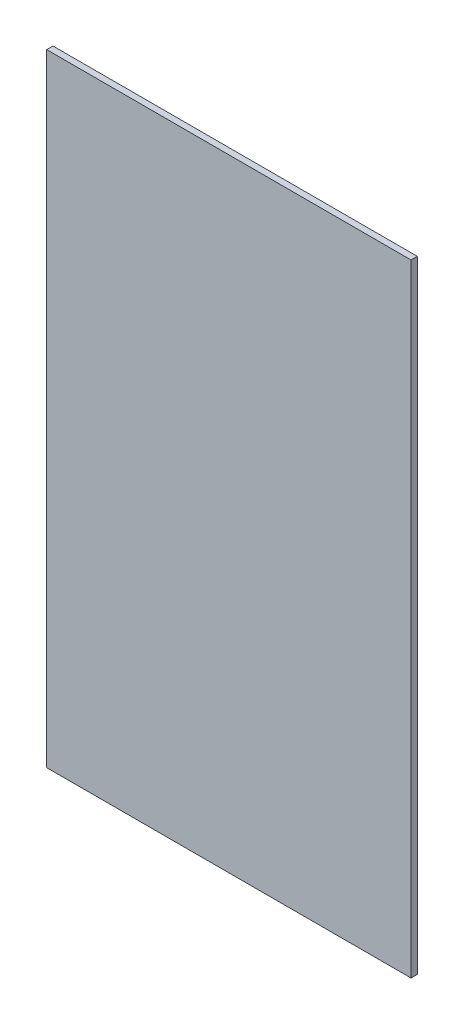
from build123d import *

# Parameters (mm, degrees)
SKETCH1_W           = 58
SKETCH1_H           = 99
BOSS_EXTRUDE1_DEPTH = 1


with BuildPart() as part:
    # Sketch1 → Boss-Extrude1 (new body)
    with BuildSketch(Plane.XY):
        Rectangle(SKETCH1_W, SKETCH1_H)
    extrude(amount=BOSS_EXTRUDE1_DEPTH)


solid = part.part
